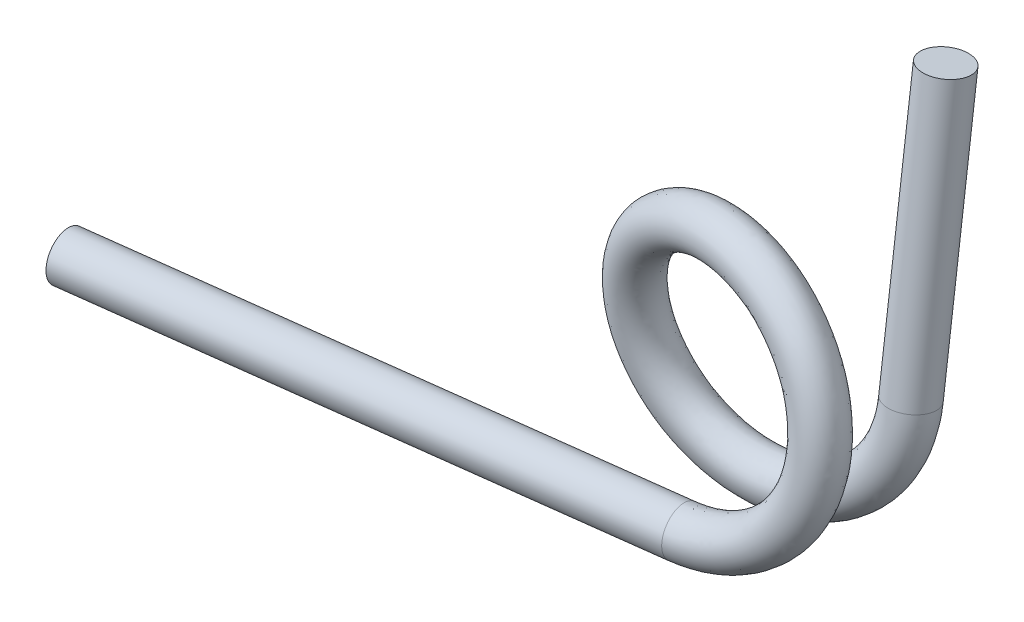
from build123d import *

# Parameters (mm, degrees)
SWEEP1_PITCH        = 2
SWEEP1_HEIGHT       = 2.5
SWEEP1_RADIUS       = 2.5
SWEEP1_PROFILE_R    = 0.5
SKETCH8_R           = 0.5
BOSS_EXTRUDE1_DEPTH = 12
SKETCH9_R           = 0.5
BOSS_EXTRUDE2_DEPTH = 6


with BuildPart() as part:
    # Sweep1: sweep along a helix
    with BuildLine() as sweep1_path:
        Helix(SWEEP1_PITCH, SWEEP1_HEIGHT, SWEEP1_RADIUS, center=(0, 0, 0), direction=(0, 0, 1), lefthand=True)
    # Sweep1 profile (on start of the path) → Sweep1 (sweep)
    with BuildSketch(Plane(origin=(2.5, 0, 0), x_dir=(0, -0.1263042864341026, -0.9919915459460187), z_dir=(1.6922325878761384e-13, -0.9919915459460187, 0.1263042864341026))):
        Circle(SWEEP1_PROFILE_R)
    sweep(path=sweep1_path.line, is_frenet=True)

    # Sketch8 → Boss-Extrude1 (add)
    with BuildSketch(Plane(origin=(-0.313231961, 0, 0.039881932), x_dir=(0.03140455580062002, 0.9685954441994059, 0.2466508044809937), z_dir=(-0.9919915459460137, 2.652392194768538e-14, 0.12630428643414296))):
        with Locations(Location((-1.804861599, -3.023701337, 0), (0, 0, 104.397169825))):
            Circle(SKETCH8_R)
    extrude(amount=BOSS_EXTRUDE1_DEPTH)

    # Sketch9 → Boss-Extrude2 (add)
    with BuildSketch(Plane(origin=(0, 0, 0), x_dir=(1, 0, 0), z_dir=(0, 0.9919915459460136, -0.12630428643414301))):
        with Locations(Location((2.5, 0, 0), (0, 0, 90))):
            Circle(SKETCH9_R)
    extrude(amount=BOSS_EXTRUDE2_DEPTH)


solid = part.part
